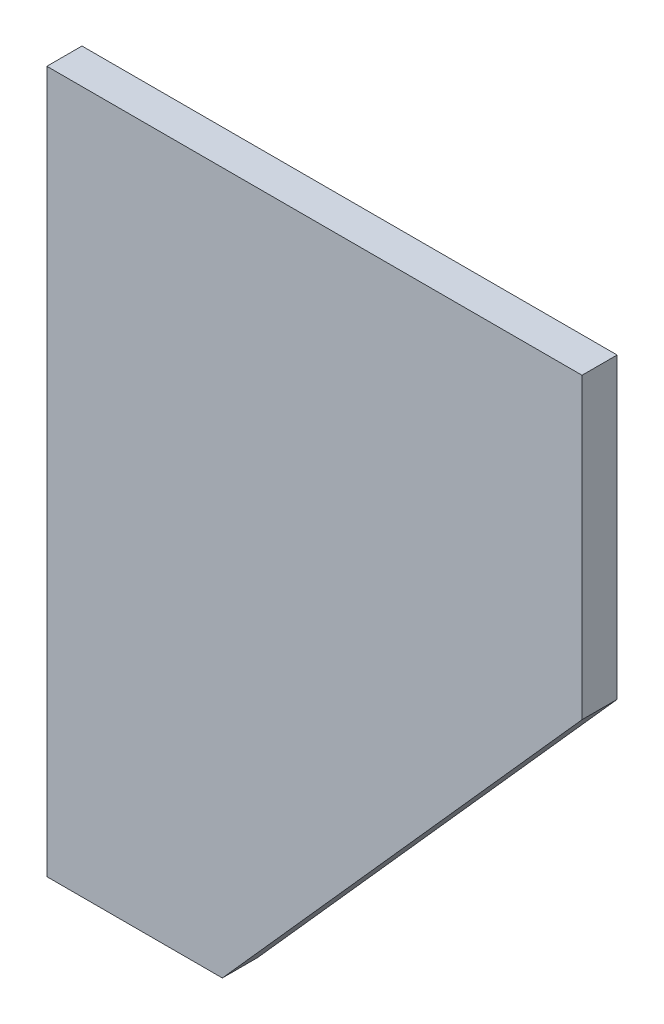
from build123d import *

# Parameters (mm, degrees)
EXTRUDE_1_DEPTH = 2


with BuildPart() as part:
    # 草图1 → 凸台-拉伸1 (new body)
    with BuildSketch(Plane.XY):
        Polygon((0, 0), (30.5, 0), (30.5, -17), (10, -40), (0, -40), align=None)
    extrude(amount=EXTRUDE_1_DEPTH)


solid = part.part
